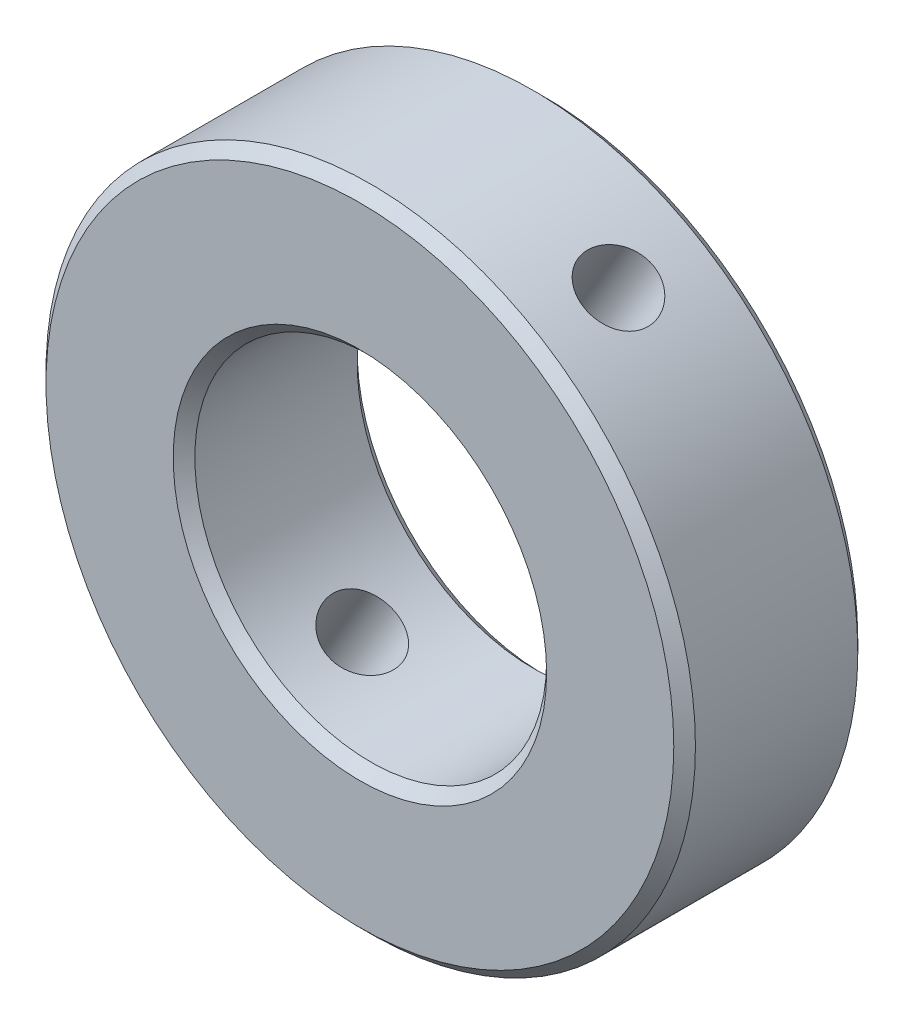
from build123d import *

# Parameters (mm, degrees)
SKETCH1_R                  = 60
SKETCH1_R_2                = 32.5
BOSS_EXTRUDE1_DEPTH        = 34
F_13_0_13_DIAMETER_HOLE1_D = 13
CHAMFER1_SIZE              = 2


with BuildPart() as part:
    # Sketch1 → Boss-Extrude1 (new body)
    with BuildSketch(Plane.XY):
        Circle(SKETCH1_R)
        Circle(SKETCH1_R_2, mode=Mode.SUBTRACT)
    extrude(amount=BOSS_EXTRUDE1_DEPTH)

    # Ø13.0 (13) Diameter Hole1 (through all)
    with Locations(Plane(origin=(30.853778368, 51.459152348, 17), x_dir=(0.85765253914, -0.514229639467, 0), z_dir=(0.514229639467, 0.85765253914, 0))):
        with Locations((0, 0)):
            Hole(F_13_0_13_DIAMETER_HOLE1_D / 2)

    # Chamfer1
    chamfer1_edges = [part.edges().sort_by_distance(p)[0] for p in [
        (-60, 0, 0),
        (-60, 0, 34),
        (-32.5, 0, 0),
        (-32.5, 0, 34),
    ]]
    chamfer(chamfer1_edges, length=CHAMFER1_SIZE)


solid = part.part
